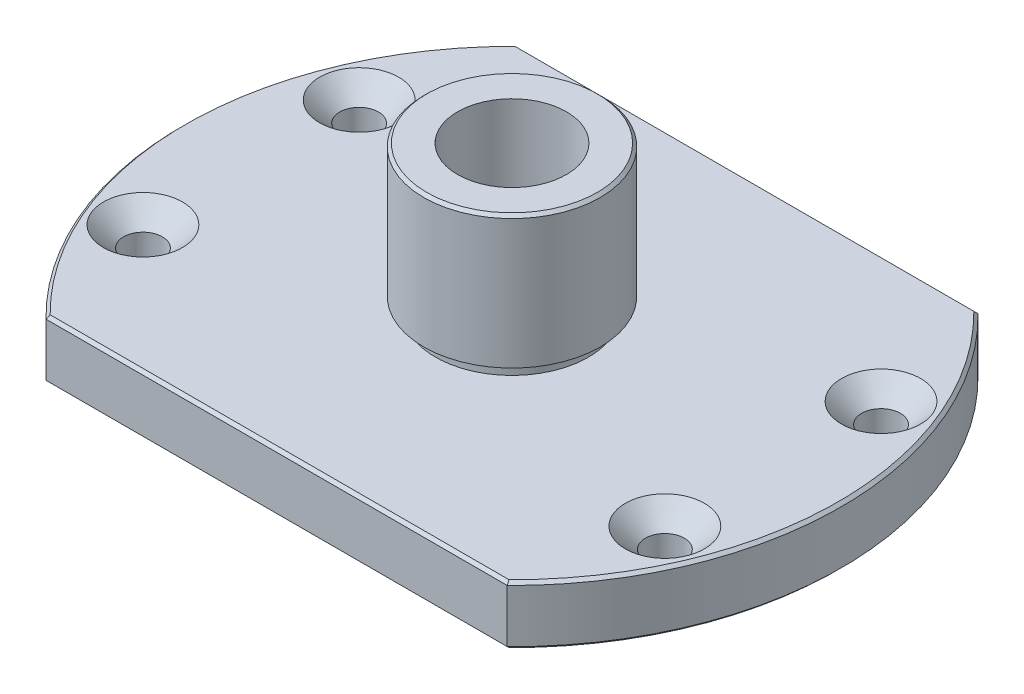
SolidWorks part; units mm, degrees
ref_plane "前视基准面" through (0, 0, 0) normal (0, 0, 1) x (1, 0, 0)
ref_plane "上视基准面" through (0, 0, 0) normal (0, 1, 0) x (1, 0, 0)
ref_plane "右视基准面" through (0, 0, 0) normal (1, 0, 0) x (0, 0, -1)
sketch "草图1" plane through (0, 0, 0) normal (0, 1, 0) x (1, 0, 0)
  circle A0 centre (0, 0) radius 56
  dimension "D1" = 112
extrude "凸台-拉伸1" add sketch "草图1" along normal blind 10
sketch "草图2" plane through (0, 10, 0) normal (0, 1, 0) x (1, 0, 0)
  circle A0 centre (0, 0) radius 15
  dimension "D1" = 30
extrude "凸台-拉伸2" add sketch "草图2" along normal blind 25
hole_wizard "M20x1.5 螺纹孔1" positions "草图4" profile "草图3" tap size "M20x1.5" standard "ISO"
sketch "草图4" plane through (0, 35, 0) normal (0, 1, 0) x (1, 0, 0)
  point P0 (0, 0)
sketch "草图3" plane through (0, 35, 0) normal (1, 0, 0) x (0, 0, 1)
  line L0 (0, 0) -> (0, 50.058)
  line L1 (0, 50.058) -> (9.25, 44.5)
  line L2 (9.25, 44.5) -> (9.25, 0)
  line L5 (9.25, 0) -> (0, 0)
  line L10 (0, 50.058) -> (-9.25, 44.5) construction
  line L11 (0, -6.35) -> (0, 107.95) construction
  dimension "螺纹孔钻头直径" = 18.5
  dimension "螺纹孔钻头深度" = 44.5
  dimension "导头角度" = 118
cosmetic thread "孔螺蚊线1" parameters "D1"=33, "D2"=20
hole_wizard "M6 六角凹锥坑螺钉的锥形沉头孔1" positions "草图11" profile "草图10" countersink size "M6" standard "ISO" end condition through all
sketch "草图11" plane through (0, 10, 0) normal (0, 1, 0) x (1, 0, 0)
  line L1 (-44.3462, 18.3688) -> (44.3462, 18.3688) construction
  line L2 (-44.3462, 18.3688) -> (-44.3462, -18.3688) construction
  line L3 (-44.3462, -18.3688) -> (44.3462, -18.3688) construction
  line L4 (44.3462, 18.3688) -> (44.3462, -18.3688) construction
  line L5 (-44.3462, 18.3688) -> (44.3462, -18.3688) construction
  line L6 (-44.3462, -18.3688) -> (44.3462, 18.3688) construction
  line L7 (0, 0) -> (52.3755, 0) construction
  circle A0 centre (0, 0) radius 48 construction
  point P6 (44.3462, -18.3688)
  point P113 (-44.3462, 18.3688)
  point P114 (-44.3462, -18.3688)
  point P115 (44.3462, 18.3688)
  dimension "D1" = 96
  dimension "D2" = 45
sketch "草图10" plane through (44.3462, 10, 18.3688) normal (1, 0, 0) x (0, 0, 1)
  line L0 (0, 0) -> (0, 10)
  line L1 (0, 10) -> (3.3, 10)
  line L2 (3.3, 10) -> (3.3, 3.42)
  line L3 (3.3, 3.42) -> (6.72, 0)
  line L5 (6.72, 0) -> (0, 0)
  line L6 (-3.3, 3.42) -> (-6.72, 0) construction
  line L11 (0, -6.35) -> (0, 107.95) construction
  dimension "通孔孔直径" = 6.6
  dimension "通孔孔深度" = 10
  dimension "近端锥形沉头孔直径" = 13.44
  dimension "近端锥形沉头孔角度" = 90
sketch "草图12" plane through (0, 10, 0) normal (0, 1, 0) x (1, 0, 0)
  line L1 (-68.0627, 40) -> (68.0627, 40)
  line L2 (-68.0627, 40) -> (-68.0627, -40)
  line L3 (-68.0627, -40) -> (68.0627, -40)
  line L4 (68.0627, 40) -> (68.0627, -40)
  line L5 (-68.0627, 40) -> (68.0627, -40) construction
  line L6 (-68.0627, -40) -> (68.0627, 40) construction
  point P0 (0, 0)
  dimension "D1" = 80
  dimension "D2" = 40
extrude "切除-拉伸1" cut sketch "草图12" against normal blind 25 flip side to cut
sketch "草图13" plane through (0, 0, 0) normal (0, 0, 1) x (1, 0, 0)
  line L0 (0, -2.7973) -> (0, 34.6576) construction
  line L1 (-15, 10) -> (-13, 10)
  line L2 (-15, 10) -> (-15, 12.5)
  line L3 (-15, 12.5) -> (-13, 12.5)
  line L4 (-13, 10) -> (-13, 12.5)
  dimension "D1" = 2
  dimension "D2" = 2.5
revolve "切除-旋转1" cut sketch "草图13" angle 360 about L0
chamfer "倒角7" distance 0.5 angle 45 9 edges at (-56, 10, 0) (56, 10, 0) (0, 10, -40) (0, 10, 40) (-56, 0, 0) (56, 0, 0) (0, 0, -40) (0, 0, 40) (0, 35, 15)
sketch "草图14" plane through (0, 0, 0) normal (0, -1, 0) x (1, 0, 0)
  circle A0 centre (0, 0) radius 15
  dimension "D1" = 30
extrude "切除-拉伸2" cut sketch "草图14" against normal blind 5
